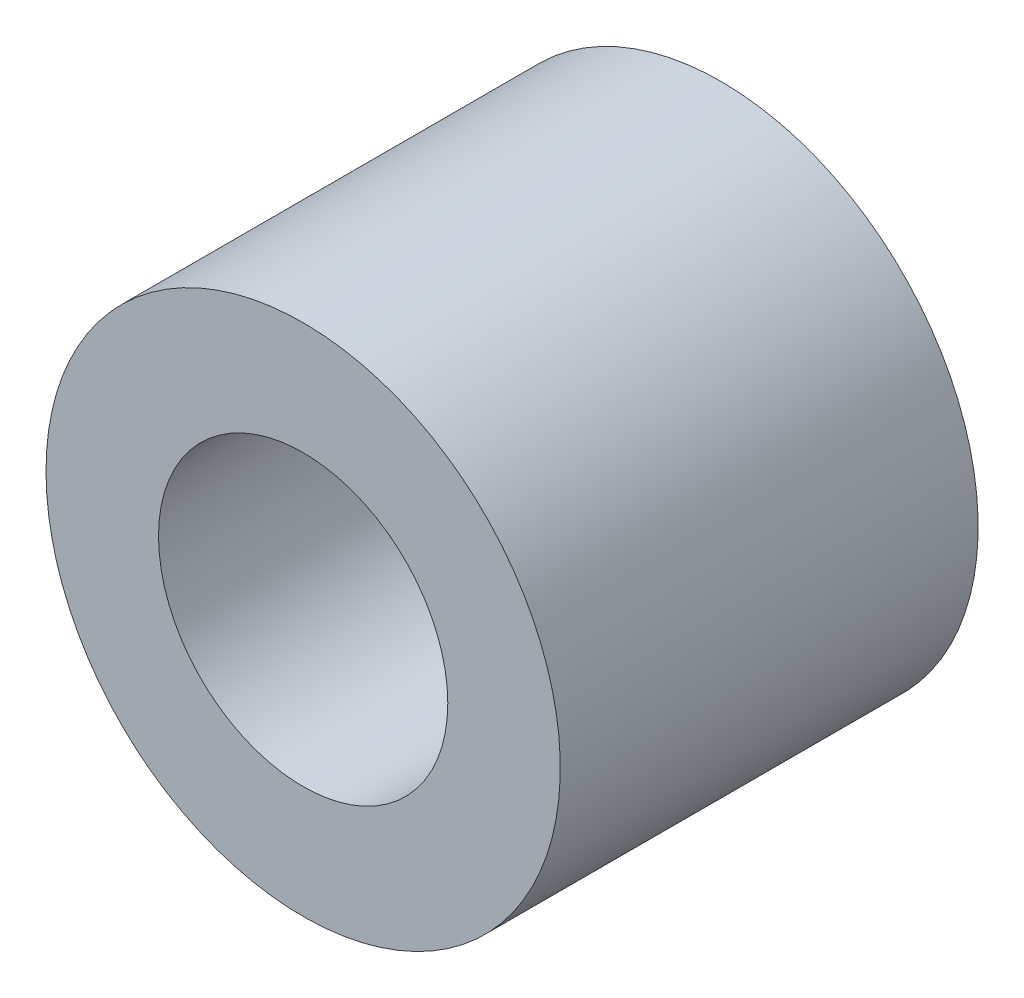
SolidWorks part; units mm, degrees
ref_plane "前视基准面" through (0, 0, 0) normal (0, 0, 1) x (1, 0, 0)
ref_plane "上视基准面" through (0, 0, 0) normal (0, 1, 0) x (1, 0, 0)
ref_plane "右视基准面" through (0, 0, 0) normal (1, 0, 0) x (0, 0, -1)
sketch "草图4" plane through (0, 0, 0) normal (0, 0, 1) x (1, 0, 0)
  circle A0 centre (0, 0) radius 4
  dimension "D1" = 8
extrude "凸台-拉伸1" add sketch "草图4" along normal blind 6.5
sketch "草图9" plane through (0, 0, 6.5) normal (0, 0, 1) x (1, 0, 0)
  circle A0 centre (0, 0) radius 2.25
  dimension "D1" = 4.5
extrude "切除-拉伸1" cut sketch "草图9" against normal through all
